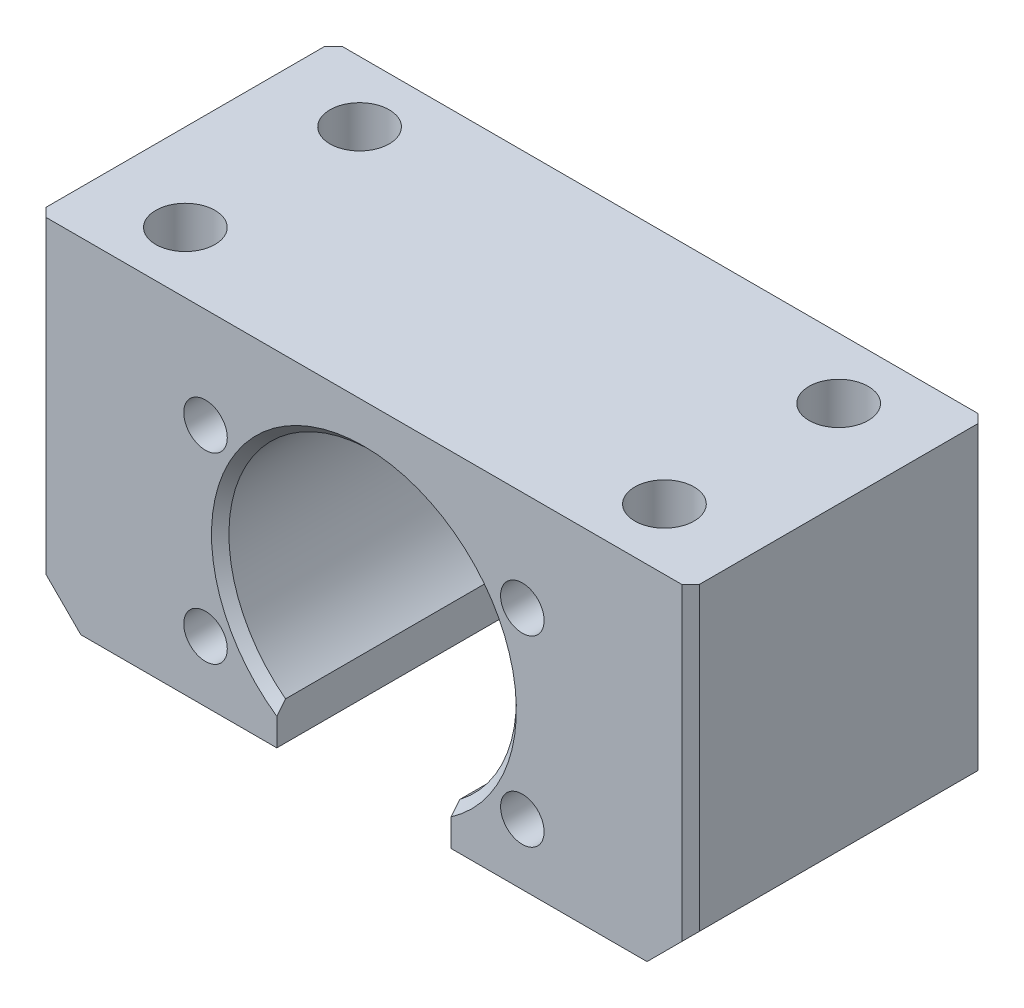
from build123d import *

# Parameters (mm, degrees)
SKETCH_1_W             = 75
SKETCH_1_H             = 39.5
EXTRUDE_1_DEPTH        = 34
SKETCH_2_R             = 16.5
CUT_EXTRUDE_1_DEPTH    = 55.335186574
SKETCH_3_W             = 20
SKETCH_3_H             = 4.375595252
CUT_EXTRUDE_2_DEPTH    = 55.335186574
HOLE_WIZARD_M8_1_D     = 6.8
HOLE_WIZARD_M8_1_DEPTH = 19.75
HOLE_WIZARD_M8_1_TIP   = 2.042926105
CHAMFER_1_SIZE         = 5
CHAMFER_2_SIZE         = 1
HOLE_WIZARD_M6_1_D     = 5
HOLE_WIZARD_M6_1_DEPTH = 15
HOLE_WIZARD_M6_1_TIP   = 1.502151548


with BuildPart() as part:
    # 草图1 → 凸台-拉伸1 (new body)
    with BuildSketch(Plane.XY):
        Rectangle(SKETCH_1_W, SKETCH_1_H)
    extrude(amount=EXTRUDE_1_DEPTH)

    # 草图2 → 切除-拉伸1 (cut, through all)
    with BuildSketch(Plane.XY.offset(34)):
        with Locations((0, -2.25)):
            Circle(SKETCH_2_R)
    extrude(amount=-CUT_EXTRUDE_1_DEPTH, mode=Mode.SUBTRACT)

    # 草图3 → 切除-拉伸2 (cut, through all)
    with BuildSketch(Plane.XY.offset(34)):
        with Locations((0, -17.562202374)):
            Rectangle(SKETCH_3_W, SKETCH_3_H)
    extrude(amount=-CUT_EXTRUDE_2_DEPTH, mode=Mode.SUBTRACT)

    # M8 螺纹孔1
    with Locations(Plane(origin=(0, 19.75, 0), x_dir=(1, 0, 0), z_dir=(0, 1, 0))):
        with Locations((-27.5, -7), (-27.5, -27), (27.5, -27), (27.5, -7)):
            Hole(HOLE_WIZARD_M8_1_D / 2, depth=HOLE_WIZARD_M8_1_DEPTH)
            with Locations((0, 0, -(HOLE_WIZARD_M8_1_DEPTH + HOLE_WIZARD_M8_1_TIP / 2))):  # 118° drill point
                Cone(0, HOLE_WIZARD_M8_1_D / 2, HOLE_WIZARD_M8_1_TIP, mode=Mode.SUBTRACT)

    # 倒角1
    chamfer_1_edges = [part.edges().sort_by_distance(p)[0] for p in [
        (37.5, -19.75, 17),
        (-37.5, -19.75, 17),
    ]]
    chamfer(chamfer_1_edges, length=CHAMFER_1_SIZE)

    # 倒角2
    chamfer_2_edges = [part.edges().sort_by_distance(p)[0] for p in [
        (-37.5, 2.5, 34),
        (0, 14.25, 0),
        (0, 14.25, 34),
        (-37.5, 2.5, 0),
        (37.5, 2.5, 0),
        (37.5, 2.5, 34),
    ]]
    chamfer(chamfer_2_edges, length=CHAMFER_2_SIZE)

    # M6 螺纹孔1
    with Locations(Plane.XY.offset(34)):
        with Locations((-18.186533479, 8.25), (-18.186533479, -12.75), (18.186533479, 8.25), (18.186533479, -12.75)):
            Hole(HOLE_WIZARD_M6_1_D / 2, depth=HOLE_WIZARD_M6_1_DEPTH)
            with Locations((0, 0, -(HOLE_WIZARD_M6_1_DEPTH + HOLE_WIZARD_M6_1_TIP / 2))):  # 118° drill point
                Cone(0, HOLE_WIZARD_M6_1_D / 2, HOLE_WIZARD_M6_1_TIP, mode=Mode.SUBTRACT)


solid = part.part
